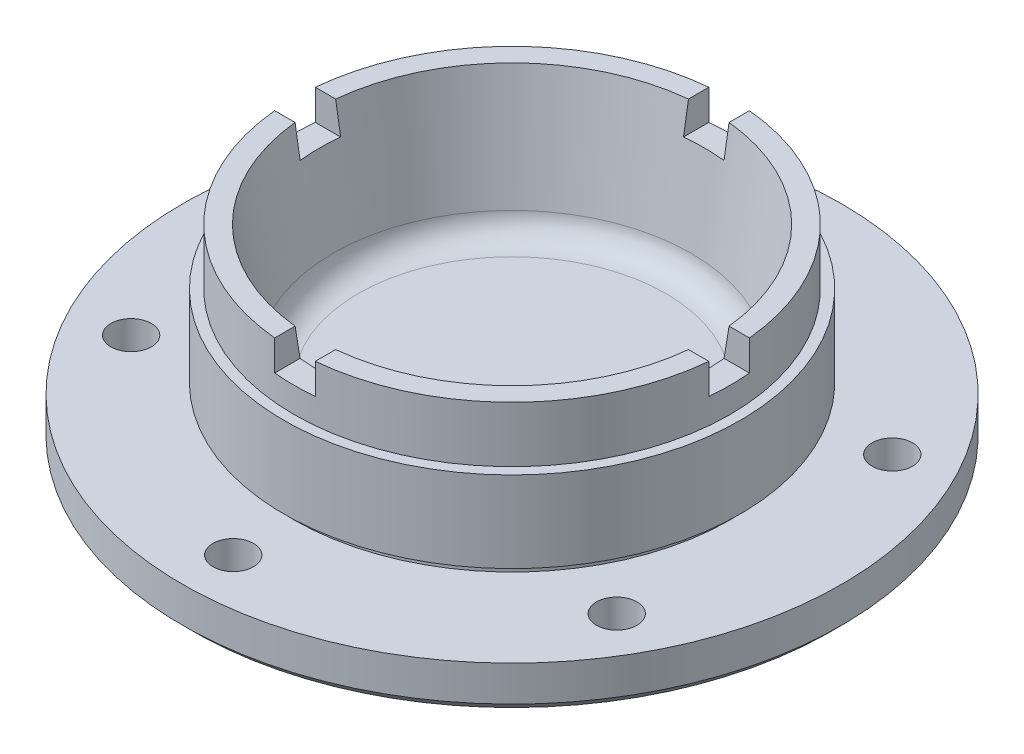
from build123d import *

# Parameters (mm, degrees)
SKETCH3_W          = 31.782249742
SKETCH3_H          = 8
SKETCH3_W_2        = 8
SKETCH3_H_2        = 31.782249742
CUT_EXTRUDE1_DEPTH = 6
CHAMFER1_SIZE      = 2
SKETCH4_R          = 4
CUT_EXTRUDE2_DEPTH = 67
SCALE_1_SCALE      = 1.875


with BuildPart() as part:
    # Sketch2 → Revolve1 (revolve)
    with BuildSketch(Plane.XY, mode=Mode.PRIVATE) as revolve1_sk:
        with BuildLine():
            Line((65, 9), (65, 0))
            Line((65, 0), (31, 0))
            Line((31, 0), (29, 2))
            Line((29, 2), (0, 2))
            Line((0, 2), (0, 11))
            Line((0, 11), (30.347168885, 11))
            ThreePointArc((30.347168885, 11), (33.667283917, 12.261439291), (35.312149528, 15.40926553))
            Line((35.312149528, 15.40926553), (39, 38))
            Line((39, 38), (43, 38))
            Line((43, 38), (43, 27))
            Line((43, 27), (45, 27))
            Line((45, 27), (45, 11))
            Line((45, 11), (43, 11))
            Line((43, 11), (43, 9))
            Line((43, 9), (65, 9))
        make_face()
    revolve(revolve1_sk.sketch.rotate(Axis((0, 2, 0), (0, 1, 0)), 90), axis=Axis((0, 2, 0), (0, 1, 0)))

    # Sketch3 → Cut-Extrude1 (cut)
    with BuildSketch(Plane(origin=(0, 38, 0), x_dir=(1, 0, 0), z_dir=(0, 1, 0))):
        with Locations((40.073271414, 0)):
            Rectangle(SKETCH3_W, SKETCH3_H)
        with Locations((0, 40.073271414)):
            Rectangle(SKETCH3_W_2, SKETCH3_H_2)
        with Locations((0, -40.073271414)):
            Rectangle(SKETCH3_W_2, SKETCH3_H_2)
        with Locations((-40.073271414, 0)):
            Rectangle(SKETCH3_W, SKETCH3_H)
    extrude(amount=-CUT_EXTRUDE1_DEPTH, mode=Mode.SUBTRACT)

    # Chamfer1
    chamfer1_edges = [part.edges().sort_by_distance(p)[0] for p in [
        (0, 0, 65),
    ]]
    chamfer(chamfer1_edges, length=CHAMFER1_SIZE)

    # Sketch4 → Cut-Extrude2 (cut)
    with BuildSketch(Plane(origin=(0, 38, 0), x_dir=(1, 0, 0), z_dir=(0, 1, 0))):
        with Locations(Location((0, 55, 0), (0, 0, 270))):
            Circle(SKETCH4_R)
        with Locations(Location((47.817664455, 27.174822282, 0), (0, 0, 270))):
            Circle(SKETCH4_R)
        with Locations(Location((-47.631397208, 27.5, 0), (0, 0, 270))):
            Circle(SKETCH4_R)
        with Locations(Location((-47.631397208, -27.5, 0), (0, 0, 270))):
            Circle(SKETCH4_R)
        with Locations(Location((0, -55, 0), (0, 0, 270))):
            Circle(SKETCH4_R)
        with Locations(Location((47.817664455, -27.174822282, 0), (0, 0, 270))):
            Circle(SKETCH4_R)
    extrude(amount=-CUT_EXTRUDE2_DEPTH, mode=Mode.SUBTRACT)


with BuildPart() as part_1:
    # Scale 1: scaled about (-0.000976977, 10.122102603, 0)
    add(part.part.scale(SCALE_1_SCALE).moved(Location((0.000854855, -8.856839778, 0))))


solid = part_1.part
